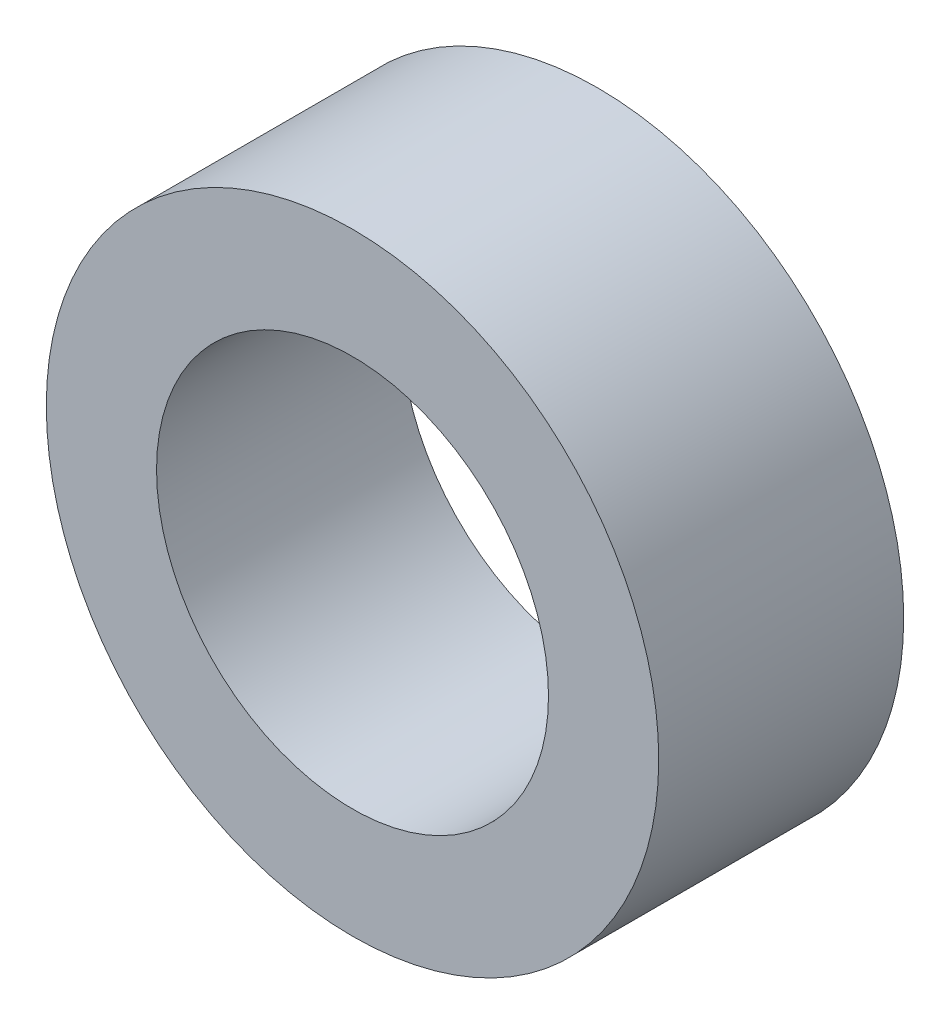
from build123d import *

# Parameters (mm, degrees)
SKETCH_1_R      = 12.5
SKETCH_1_R_2    = 8
EXTRUDE_1_DEPTH = 5


with BuildPart() as part:
    # 草图1 → 凸台-拉伸1 (new, symmetric)
    with BuildSketch(Plane.XY):
        Circle(SKETCH_1_R)
        Circle(SKETCH_1_R_2, mode=Mode.SUBTRACT)
    extrude(amount=EXTRUDE_1_DEPTH, both=True)


solid = part.part
